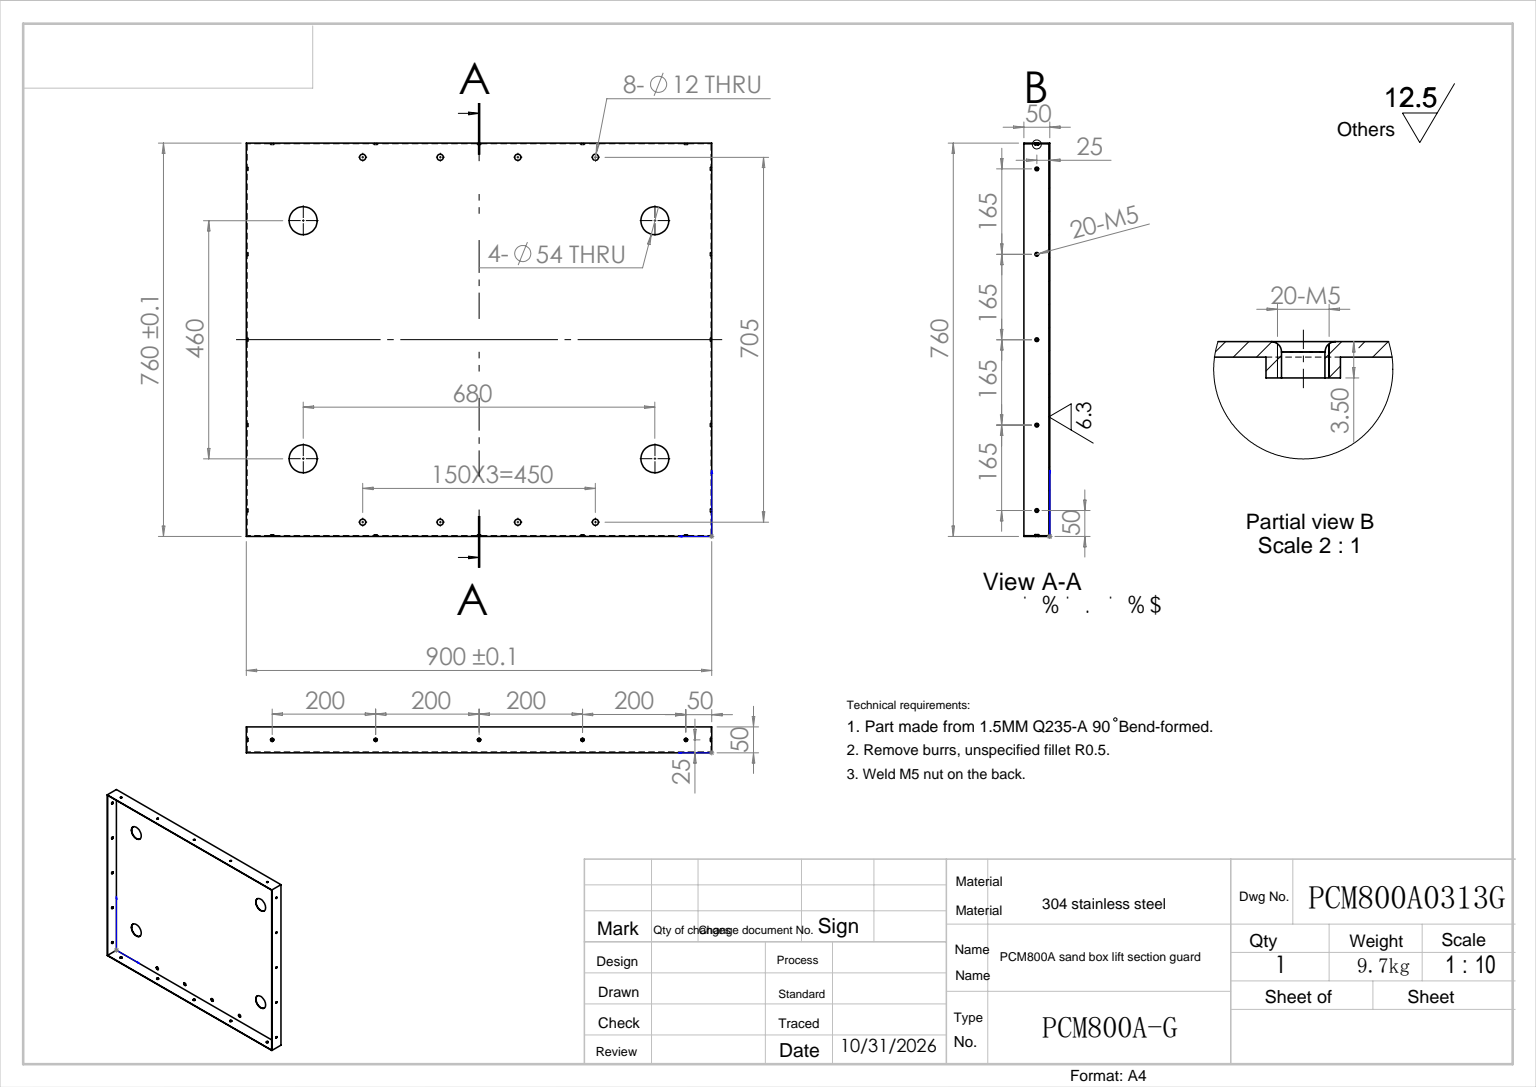
SolidWorks part; units mm, degrees
ref_plane "前视基准面" through (0, 0, 0) normal (0, 0, 1) x (1, 0, 0)
ref_plane "上视基准面" through (0, 0, 0) normal (0, 1, 0) x (1, 0, 0)
ref_plane "右视基准面" through (0, 0, 0) normal (1, 0, 0) x (0, 0, -1)
sketch "草图1" plane through (0, 0, 0) normal (0, 0, 1) x (1, 0, 0)
  line L1 (0, 0) -> (900, 0)
  line L2 (0, 0) -> (0, 760)
  line L3 (0, 760) -> (900, 760)
  line L4 (900, 0) -> (900, 760)
  dimension "D1" = 760
  dimension "D2" = 900
extrude "拉伸1" add sketch "草图1" along normal blind 50
shell "抽壳1" thickness 1.5
sketch "草图2" plane through (0, 0, 0) normal (0, 0, -1) x (-1, 0, 0)
  line L0 (0, 760) -> (0, 0) construction
  line L1 (0, 0) -> (-900, 0) construction
  circle A0 centre (-790, 610) radius 27
  circle A1 centre (-110, 610) radius 27
  circle A2 centre (-790, 150) radius 27
  circle A3 centre (-110, 150) radius 27
  dimension "D1" = 460
  dimension "D2" = 460
  dimension "D3" = 680
  dimension "D4" = 680
  dimension "D5" = 110
  dimension "D6" = 150
  dimension "D7" = 150
  dimension "D8" = 110
extrude "切除-拉伸1" cut sketch "草图2" against normal through all
sketch "草图3" plane through (0, 0, 0) normal (0, 0, -1) x (-1, 0, 0)
  circle A0 centre (-675, 732.5) radius 6
  circle A1 centre (-525, 732.5) radius 6
  circle A2 centre (-375, 732.5) radius 6
  circle A3 centre (-225, 732.5) radius 6
extrude "切除-拉伸3" cut sketch "草图3" against normal through all
ref_plane "基准面1" through (0, 380, 0) normal (0, 1, 0) x (-1, 0, 0)
mirror "镜向1" about plane through (0, 380, 0) normal (0, 1, 0) of "切除-拉伸3"
sketch "草图6" plane through (0, 1.5, 0) normal (0, 1, 0) x (1, 0, 0)
  line L0 (0, -25) -> (924.148, -25) construction
  line L1 (0, -50) -> (0, 0) construction
  line L5 (200, -25) -> (1124.148, -25) construction
  line L6 (400, -25) -> (1324.148, -25) construction
  line L7 (600, -25) -> (1524.148, -25) construction
  line L8 (800, -25) -> (1724.148, -25) construction
  circle A0 centre (50, -25) radius 3.6
  circle A4 centre (250, -25) radius 3.6
  circle A5 centre (450, -25) radius 3.6
  circle A6 centre (650, -25) radius 3.6
  circle A7 centre (850, -25) radius 3.6
  dimension "D1" = 7.2
  dimension "D2" = 50
  dimension "D3" = 5
extrude "凸台-拉伸1" add sketch "草图6" along normal blind 2
sketch "草图7" plane through (0, 758.5, 0) normal (0, -1, 0) x (1, 0, 0)
  circle A7 centre (50, 25) radius 3.6
  circle A8 centre (50, 25) radius 3.6
  circle A10 centre (250, 25) radius 3.6
  circle A11 centre (250, 25) radius 3.6
  circle A13 centre (450, 25) radius 3.6
  circle A14 centre (450, 25) radius 3.6
  circle A16 centre (650, 25) radius 3.6
  circle A17 centre (650, 25) radius 3.6
  circle A19 centre (850, 25) radius 3.6
  circle A20 centre (850, 25) radius 3.6
  dimension "D1" = 0
  dimension "D2" = 0
  dimension "D3" = 0
  dimension "D4" = 0
  dimension "D5" = 0
extrude "凸台-拉伸2" add sketch "草图7" along normal blind 2
hole_wizard "M5 螺纹孔1" positions "草图9" profile "草图8" tap size "M5" standard "GB" end condition through all
sketch "草图9" plane through (0, 0, 0) normal (0, -1, 0) x (1, 0, 0)
  point P1 (50, 25)
  point P4 (250, 25)
  point P7 (450, 25)
  point P10 (650, 25)
  point P13 (850, 25)
cosmetic thread "孔螺蚊线1" parameters "D2"=5
cosmetic thread "孔螺蚊线2" parameters "D2"=5
cosmetic thread "孔螺蚊线3" parameters "D2"=5
cosmetic thread "孔螺蚊线4" parameters "D2"=5
cosmetic thread "孔螺蚊线5" parameters "D2"=5
sketch "草图8" plane through (50, 0, 25) normal (1, 0, 0) x (0, 0, -1)
  line L0 (0, 0) -> (0, 760)
  line L1 (0, 760) -> (2.1, 760)
  line L2 (2.1, 760) -> (2.1, 0)
  line L5 (2.1, 0) -> (0, 0)
  line L11 (0, -6.35) -> (0, 107.95) construction
  dimension "通孔螺纹孔钻头直径" = 4.2
  dimension "通孔螺纹孔钻头深度" = 760
sketch "草图10" plane through (1.5, 0, 0) normal (1, 0, 0) x (0, 0, -1)
  line L0 (-25, 760) -> (-25, -93.648) construction
  line L1 (-50, 760) -> (0, 760) construction
  circle A0 centre (-25, 710) radius 3.6
  circle A1 centre (-25, 545) radius 3.6
  circle A2 centre (-25, 380) radius 3.6
  circle A3 centre (-25, 215) radius 3.6
  circle A4 centre (-25, 50) radius 3.6
  dimension "D1" = 7.2
  dimension "D2" = 50
  dimension "D3" = 5
extrude "凸台-拉伸3" add sketch "草图10" along normal blind 2
sketch "草图11" plane through (898.5, 0, 0) normal (-1, 0, 0) x (0, 0, 1)
  circle A2 centre (25, 710) radius 3.6
  circle A3 centre (25, 710) radius 3.6
  circle A5 centre (25, 545) radius 3.6
  circle A6 centre (25, 545) radius 3.6
  circle A8 centre (25, 380) radius 3.6
  circle A9 centre (25, 380) radius 3.6
  circle A11 centre (25, 215) radius 3.6
  circle A12 centre (25, 215) radius 3.6
  circle A14 centre (25, 50) radius 3.6
  circle A15 centre (25, 50) radius 3.6
  dimension "D1" = 0
  dimension "D2" = 0
  dimension "D3" = 0
  dimension "D4" = 0
  dimension "D5" = 0
extrude "凸台-拉伸4" add sketch "草图11" along normal blind 2
hole_wizard "M5 螺纹孔2" positions "草图13" profile "草图12" tap size "M5" standard "GB" end condition through all
sketch "草图13" plane through (900, 0, 0) normal (1, 0, 0) x (0, 0, -1)
  point P1 (-25, 710)
  point P4 (-25, 545)
  point P7 (-25, 380)
  point P10 (-25, 215)
  point P13 (-25, 50)
cosmetic thread "孔螺蚊线6" parameters "D2"=5
cosmetic thread "孔螺蚊线7" parameters "D2"=5
cosmetic thread "孔螺蚊线8" parameters "D2"=5
cosmetic thread "孔螺蚊线9" parameters "D2"=5
cosmetic thread "孔螺蚊线10" parameters "D2"=5
sketch "草图12" plane through (900, 710, 25) normal (0, 1, 0) x (0, 0, -1)
  line L0 (0, 0) -> (0, 900)
  line L1 (0, 900) -> (2.1, 900)
  line L2 (2.1, 900) -> (2.1, 0)
  line L5 (2.1, 0) -> (0, 0)
  line L11 (0, -6.35) -> (0, 107.95) construction
  dimension "通孔螺纹孔钻头直径" = 4.2
  dimension "通孔螺纹孔钻头深度" = 900
fillet "圆角1" radius 1 20 edges at (250, 760, 22.9) (50, 760, 22.9) (0, 710, 22.9) (900, 710, 22.9) (900, 545, 22.9) (900, 380, 22.9) (900, 215, 22.9) (900, 50, 22.9) (850, 0, 22.9) (650, 0, 22.9) (450, 0, 22.9) (250, 0, 22.9) (50, 0, 22.9) (0, 50, 22.9) (0, 215, 22.9) (0, 380, 22.9) (0, 545, 22.9) (850, 760, 22.9) (650, 760, 22.9) (450, 760, 22.9)
